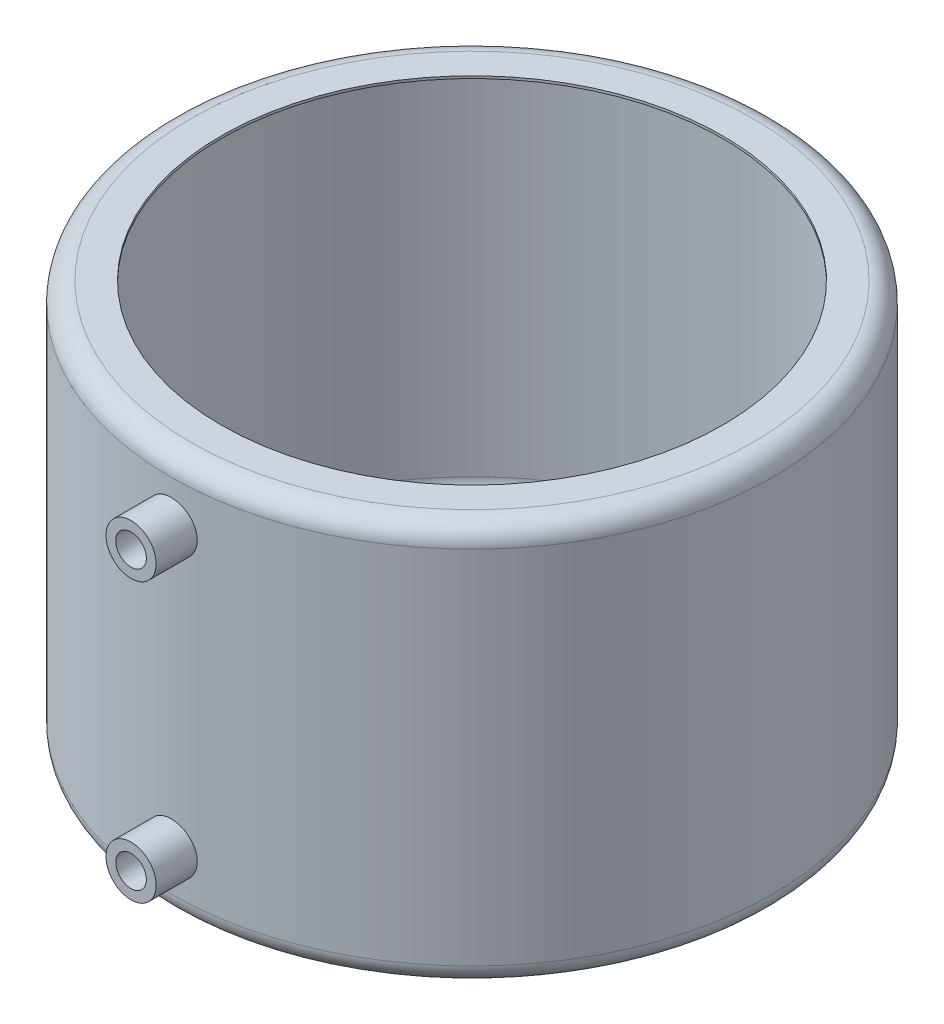
SolidWorks part; units mm, degrees
material "AISI 304"
ref_plane "Front Plane" through (0, 0, 0) normal (0, 0, 1) x (1, 0, 0)
ref_plane "Top Plane" through (0, 0, 0) normal (0, 1, 0) x (1, 0, 0)
ref_plane "Right Plane" through (0, 0, 0) normal (1, 0, 0) x (0, 0, -1)
sketch "Sketch1" plane through (0, 0, 0) normal (0, 1, 0) x (1, 0, 0)
  circle A0 centre (0, 0) radius 150
  dimension "D1" = 300
extrude "Boss-Extrude1" add sketch "Sketch1" along normal blind 200
fillet "Fillet1" radius 10 2 edges at (0, 0, 150) (0, 200, 150)
sketch "Sketch2" plane through (0, 200, 0) normal (0, 1, 0) x (1, 0, 0)
  circle A0 centre (0, 0) radius 125
  dimension "D1" = 250
extrude "Cut-Extrude1" cut sketch "Sketch2" against normal through all
shell "Shell2" thickness 1.2
ref_plane "Plane1" through (0, 0, 170) normal (0, 0, 1) x (1, 0, 0)
sketch "Sketch5" plane through (0, 0, 170) normal (0, 0, 1) x (1, 0, 0)
  line L0 (-125, 198.8) -> (125, 198.8) construction
  circle A0 centre (0, 30) radius 12.5
  circle A1 centre (0, 168.8) radius 12.5
  dimension "D1" = 25
  dimension "D3" = 30
  dimension "D2" = 30
extrude "Boss-Extrude2" add sketch "Sketch5" against normal up to surface (21.726 mm away)
hole_wizard "G3/8 Tapped Hole1" positions "3DSketch1" profile "Sketch6" tap size "G3/8" standard "GB"
sketch3d "3DSketch1"
  line L0 (0, 30, 149.4783) -> (0, 30, 170) construction
  line L1 (0, 168.8, 149.4783) -> (0, 168.8, 170) construction
  point P0 (0, 30, 170)
  point P5 (0, 168.8, 170)
sketch "Sketch6" plane through (0, 30, 170) normal (1, 0, 0) x (0, -1, 0)
  line L0 (0, 0) -> (0, 41.9116)
  line L1 (0, 41.9116) -> (7.625, 37.33)
  line L2 (7.625, 37.33) -> (7.625, 0)
  line L5 (7.625, 0) -> (0, 0)
  line L10 (0, 41.9116) -> (-7.625, 37.33) construction
  line L11 (0, -6.35) -> (0, 107.95) construction
  dimension "螺纹孔钻头直径" = 15.25
  dimension "螺纹孔钻头深度" = 37.33
  dimension "导头角度" = 118
cosmetic thread "CosmeticThread Thread1" parameters "D1"=21.1952, "D2"=16.662
cosmetic thread "CosmeticThread Thread2" parameters "D1"=21.1952, "D2"=16.662
